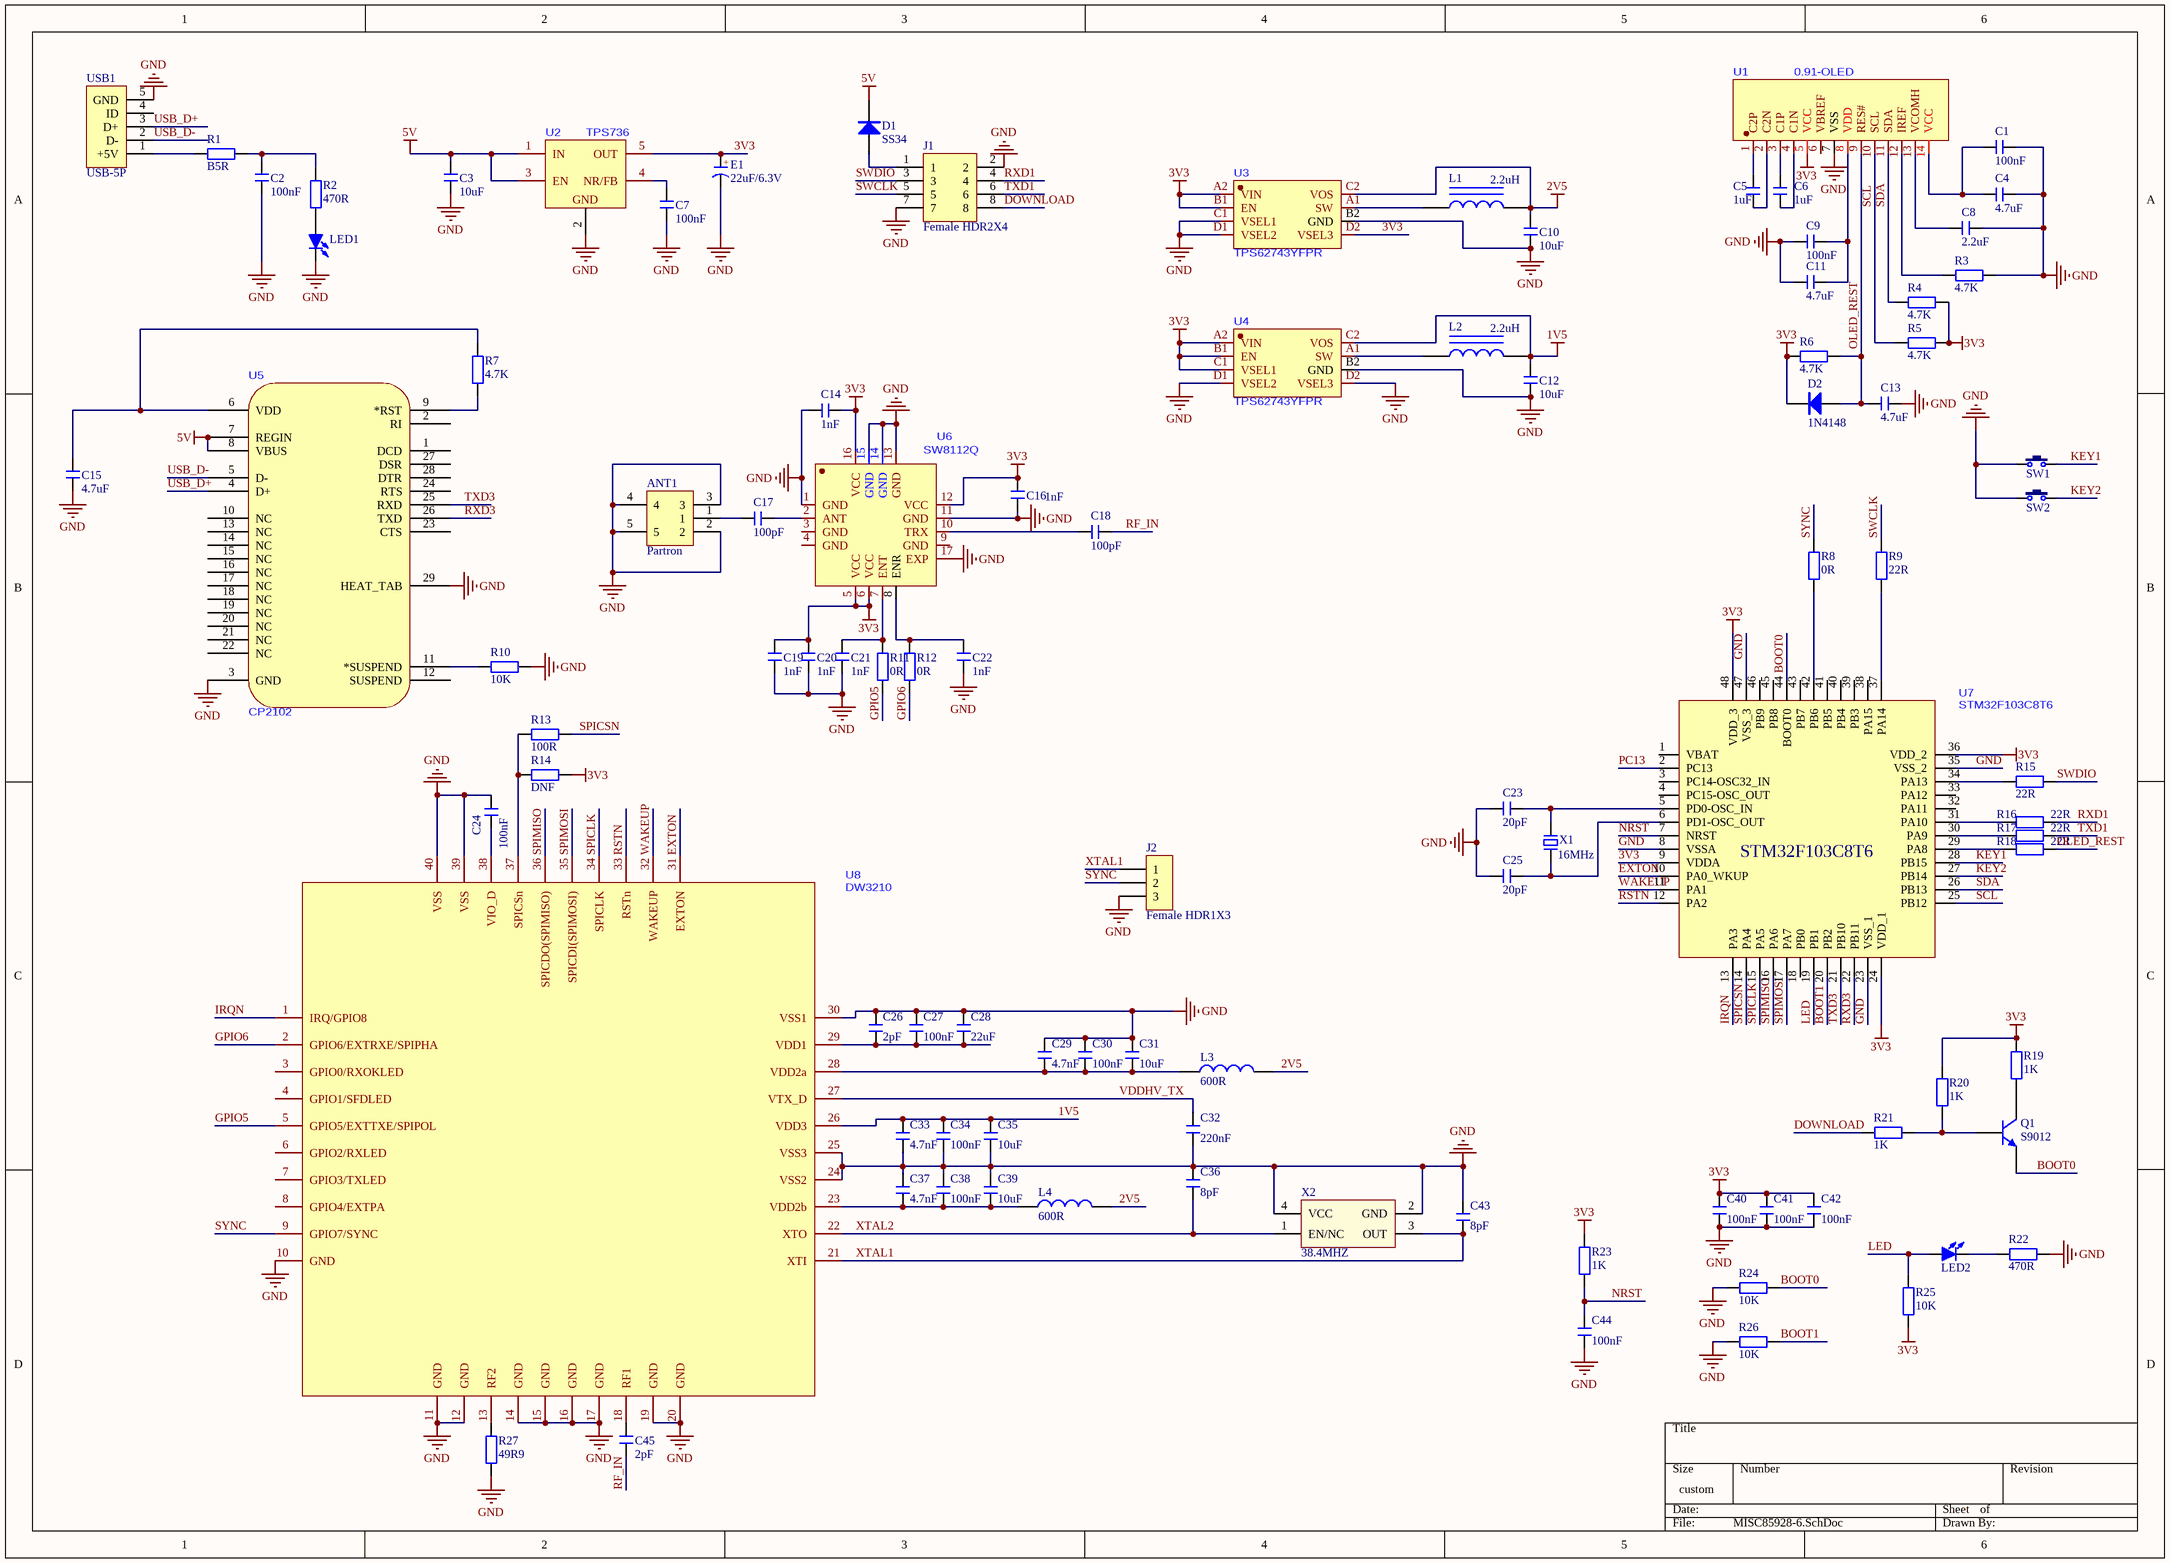
[diagram p0: MISC85928-6.SchDoc]
# Altium project MISC85928-2.PrjPcb
1 sheet, 98 parts. Net scope: global (net labels, ports and power ports of the same name join across sheets).
Board file: MISC85928.PcbDoc

## Sheet MISC85928-6.SchDoc
size 406 x 292 mm

### Parts
ANT1  Partron  [天线座5p]
C1  100nF  [C 0603_L]
C2  100nF  [C 0603_L]
C3  10uF  [C 0603_L]
C4  4.7uF  [C 0603_L]
C5  1uF  [C 0603_L]
C6  1uF  [C 0603_L]
C7  100nF  [C 0603_L]
C8  2.2uF  [C 0603_L]
C9  100nF  [C 0603_L]
C10  10uF  [C 0603_L]
C11  4.7uF  [C 0603_L]
C12  10uF  [C 0603_L]
C13  4.7uF  [C 0603_L]
C14  1nF  [C 0603_L]
C15  4.7uF  [C 0603_L]
C16  1nF  [C 0603_L]
C17  100pF  [C 0603_L]
C18  100pF  [C 0603_L]
C19  1nF  [C 0603_L]
C20  1nF  [C 0603_L]
C21  1nF  [C 0603_L]
C22  1nF  [C 0603_L]
C23  20pF  [C 0603_L]
C24  100nF  [C 0603_L]
C25  20pF  [C 0603_L]
C26  2pF  [C 0603_L]
C27  100nF  [C 0603_L]
C28  22uF  [C 0603_L]
C29  4.7nF  [C 0603_L]
C30  100nF  [C 0603_L]
C31  10uF  [C 0603_L]
C32  220nF  [C 0603_L]
C33  4.7nF  [C 0603_L]
C34  100nF  [C 0603_L]
C35  10uF  [C 0603_L]
C36  8pF  [C 0603_L]
C37  4.7nF  [C 0603_L]
C38  100nF  [C 0603_L]
C39  10uF  [C 0603_L]
C40  100nF  [C 0603_L]
C41  100nF  [C 0603_L]
C42  100nF  [C 0603_L]
C43  8pF  [C 0603_L]
C44  100nF  [C 0603_L]
C45  2pF  [C 0603_L]
D1  SS34  [MINI_MELF (LL34)]
D2  1N4148  [MINI_MELF (LL34)]
E1  22uF/6.3V  [C 0603_L]
J1  Female HDR2X4  [Fe-HDR2X4/2.54-S]
J2  Female HDR1X3  [Fe-HDR1X3/2.54-S]
L1  value 2.2uH  [L 0603]  (hidden comment: Inductor Iron)
L2  value 2.2uH  [L 0603]  (hidden comment: Inductor Iron)
L3  600R  [L 0603]
L4  600R  [L 0603]
LED1  Red  [LED 0805G]  (value not drawn)
LED2  Red  [LED 0805G]  (value not drawn)
Q1  S9012  [SOT-23B_N]
R1  B5R  [R 0603_L]
R2  470R  [R 0603_L]
R3  4.7K  [R 0603_L]
R4  4.7K  [R 0603_L]
R5  4.7K  [R 0603_L]
R6  4.7K  [R 0603_L]
R7  4.7K  [R 0603_L]
R8  0R  [R 0603_L]
R9  22R  [R 0603_L]
R10  10K  [R 0603_L]
R11  0R  [R 0603_L]
R12  0R  [R 0603_L]
R13  100R  [R 0603_L]
R14  DNF  [R 0603_L]
R15  22R  [R 0603_L]
R16  22R  [R 0603_L]
R17  22R  [R 0603_L]
R18  22R  [R 0603_L]
R19  1K  [R 0603_L]
R20  1K  [R 0603_L]
R21  1K  [R 0603_L]
R22  470R  [R 0603_L]
R23  1K  [R 0603_L]
R24  10K  [R 0603_L]
R25  10K  [R 0603_L]
R26  10K  [R 0603_L]
R27  49R9  [R 0603_L]
SW1  3x6x5  [TSW SMD-3*6*2.5]  (value not drawn)
SW2  3x6x5  [TSW SMD-3*6*2.5]  (value not drawn)
U1  0.91-OLED  [OLED0.91]
U2  TPS736  [SOT-23-5_L3.0-W1.7-P0.95-LS2.8-BR]
U3  TPS62743YFPR  [DSBGA-8_L1.6-W0.9-R2-C4-P0.40-BL]
U4  TPS62743YFPR  [DSBGA-8_L1.6-W0.9-R2-C4-P0.40-BL]
U5  CP2102  [CP2102]
U6  SW8112Q  [QFN-16_L3.0-W3.0-P0.50-BL-EP1.7]
U7  STM32F103C8T6  [LQFP48 7X7]
U8  DW3210  [DW3210]
USB1  USB-5P  [USB-MICRO_A]
X1  16MHz  [OSC 3215-2P]
X2  38.4MHZ  [OSC 1612-4P]

### Nets
1V5: C12.2 C33.1 C34.1 C35.1 L2.2 U4.C2(VOS) U8.26(VDD3)
2V5: C10.2 L1.2 L3.2 L4.2 U3.C2(VOS)
3V3: C14.1 C16.1 C19.1 C20.1 C40.1 C41.1 C42.1 D2.2(K) E1.1(A) R4.1 R5.1 R6.2 R14.1 R19.1 R20.1 R23.2 R25.2 U1.5(VCC) U2.5(OUT) U3.A2(VIN) U3.B1(EN) U3.D2(VSEL3) U4.A2(VIN) U4.B1(EN) U4.C1(VSEL1) U6.5(VCC) U6.6(VCC) U6.12(VCC) U6.16(VCC) U7.9(VDDA) U7.24(VDD_1) U7.36(VDD_2) U7.48(VDD_3)
5V: C3.2 D1.2(K) U2.1(IN) U2.3(EN) U5.7(REGIN) U5.8(VBUS)
GND: ANT1.2 ANT1.3 ANT1.4 ANT1.5 C1.1 C2.1 C3.1 C4.1 C7.1 C8.1 C9.2 C10.1 C11.2 C12.1 C13.1 C14.2 C15.1 C16.2 C19.2 C20.2 C21.2 C22.2 C23.1 C24.1 C25.1 C26.1 C27.1 C28.1 C29.1 C30.1 C31.1 C32.2 C33.2 C34.2 C35.2 C36.1 C37.1 C38.1 C39.1 C40.2 C41.2 C42.2 C43.1 C44.2 E1.2(K) J1.2 J1.7 J2.3 LED1.2(K) R3.1 R10.1 R22.2 R24.2 R26.2 R27.1 SW1.1 SW2.1 U1.7(VSS) U2.2(GND) U3.B2(GND) U3.C1(VSEL1) U3.D1(VSEL2) U4.B2(GND) U4.D1(VSEL2) U4.D2(VSEL3) U5.3(GND) U5.29(HEAT_TAB) U6.1(GND) U6.11(GND) U6.13(GND) U6.14(GND) U6.15(GND) U6.17(EXP) U7.8(VSSA) U7.23(VSS_1) U7.35(VSS_2) U7.47(VSS_3) U8.10(GND) U8.11(GND) U8.12(GND) U8.14(GND) U8.15(GND) U8.16(GND) U8.17(GND) U8.19(GND) U8.20(GND) U8.24(VSS2) U8.25(VSS3) U8.30(VSS1) U8.39(VSS) U8.40(VSS) USB1.5(GND) X2.2(GND) X2.4(VCC)
BOOT0: Q1.3(E) R24.1 U7.44(BOOT0)
BOOT1: R26.1 U7.20(PB2)
DOWNLOAD: J1.8 R21.1
EXTON: U7.10(PA0_WKUP) U8.31(EXTON)
GPIO5: R11.1 U8.5(GPIO5/EXTTXE/SPIPOL)
GPIO6: R12.1 U8.2(GPIO6/EXTRXE/SPIPHA)
IRQN: U7.13(PA3) U8.1(IRQ/GPIO8)
KEY1: SW1.2 U7.28(PB15)
KEY2: SW2.2 U7.27(PB14)
LED: LED2.1(A) R25.1 U7.19(PB1)
NRST: C44.1 R23.1 U7.7(NRST)
OLED_REST: C13.2 D2.1(A) R6.1 R18.1 U1.9(RES#)
PC13: U7.2(PC13)
RF_IN: C18.1 C45.2
RSTN: U7.12(PA2) U8.33(RSTn)
RXD1: J1.4 R16.1
RXD3: U5.26(TXD) U7.22(PB11)
SCL: R5.2 U1.10(SCL) U7.25(PB12)
SDA: R4.2 U1.11(SDA) U7.26(PB13)
SPICLK: U7.15(PA5) U8.34(SPICLK)
SPICSN: R13.1 U7.14(PA4)
SPIMISO: U7.16(PA6) U8.36(SPICDO(SPIMISO))
SPIMOSI: U7.17(PA7) U8.35(SPICDI(SPIMOSI))
SWCLK: J1.5 R9.2
SWDIO: J1.3 R15.1
SYNC: J2.2 R8.2 U8.9(GPIO7/SYNC)
TXD1: J1.6 R17.1
TXD3: U5.25(RXD) U7.21(PB10)
USB_D+: U5.4(D+) USB1.3(D+)
USB_D-: U5.5(D-) USB1.2(D-)
VDDHV_TX: C32.1 U8.27(VTX_D)
WAKEUP: U7.11(PA1) U8.32(WAKEUP)
XTAL1: C43.2 J2.1 U8.21(XTI) X2.3(OUT)
XTAL2: C36.2 U8.22(XTO) X2.1(EN/NC)
NetANT1_1: ANT1.1 C17.2
NetC1_2: C1.2 C4.2 U1.14(VCC)
NetC2_2: C2.2 R1.2 R2.2
NetC5_1: C5.1 U1.2(C2N)
NetC5_2: C5.2 U1.1(C2P)
NetC6_1: C6.1 U1.4(C1N)
NetC6_2: C6.2 U1.3(C1P)
NetC7_2: C7.2 U2.4(NR/FB)
NetC8_2: C8.2 U1.13(VCOMH)
NetC9_1: C9.1 C11.1 U1.8(VDD)
NetC15_2: C15.2 R7.2 U5.6(VDD)
NetC17_1: C17.1 U6.2(ANT)
NetC18_2: C18.2 U6.10(TRX)
NetC21_1: C21.1 R11.2 U6.7(ENT)
NetC22_1: C22.1 R12.2 U6.8(ENR)
NetC23_2: C23.2 U7.5(PD0-OSC_IN) X1.2
NetC24_2: C24.2 U8.38(VIO_D)
NetC25_2: C25.2 U7.6(PD1-OSC_OUT) X1.1
NetC26_2: C26.2 C27.2 C28.2 U8.29(VDD1)
NetC29_2: C29.2 C30.2 C31.2 L3.1 U8.28(VDD2a)
NetC37_2: C37.2 C38.2 C39.2 L4.1 U8.23(VDD2b)
NetC45_1: C45.1 U8.18(RF1)
NetD1_1: D1.1(A) J1.1
NetL1_1: L1.1 U3.A1(SW)
NetL2_1: L2.1 U4.A1(SW)
NetLED1_1: LED1.1(A) R2.1
NetLED2_2: LED2.2(K) R22.1
NetQ1_1: Q1.1(C) R19.2
NetQ1_2: Q1.2(B) R20.2 R21.2
NetR1_1: R1.1 USB1.1(+5V)
NetR3_2: R3.2 U1.12(IREF)
NetR7_1: R7.1 U5.9(*RST)
NetR8_1: R8.1 U7.42(PB6)
NetR9_1: R9.1 U7.37(PA14)
NetR10_2: R10.2 U5.11(*SUSPEND)
NetR13_2: R13.2 R14.2 U8.37(SPICSn)
NetR15_2: R15.2 U7.34(PA13)
NetR16_2: R16.2 U7.31(PA10)
NetR17_2: R17.2 U7.30(PA9)
NetR18_2: R18.2 U7.29(PA8)
NetR27_2: R27.2 U8.13(RF2)

Not connected (* = marked no-connect by the designer): U1 6(VBREF); U5 1(DCD) 2(RI) 10(NC) 12(SUSPEND) 13(NC) 14(NC) 15(NC) 16(NC) 17(NC) 18(NC) 19(NC) 20(NC) 21(NC) 22(NC) 23(CTS) 24(RTS) 27(DSR) 28(DTR); U6 3(GND) 4(GND) 9(GND); U7 1(VBAT) 3(PC14-OSC32_IN) 4(PC15-OSC_OUT) 18(PB0) 32(PA11) 33(PA12) 38(PA15) 39(PB3) 40(PB4) 41(PB5) 43(PB7) 45(PB8) 46(PB9); U8 3(GPIO0/RXOKLED) 4(GPIO1/SFDLED) 6(GPIO2/RXLED) 7(GPIO3/TXLED) 8(GPIO4/EXTPA); USB1 4(ID)

### Library data of the parts
C1-C45 = C: Chip capacitor; BOM名称: Non-polar chip capacitor
D1 D2 = 1N4148: Switching diode; BOM名称: High-speed switching diode
E1 = CT: Chip tantalum capacitor; BOM名称: Chip tantalum capacitor
L1 L2 = Inductor Iron: Magnetic-Core Inductor; Published: 24-Mar-1999; LatestRevisionDate: 17-Jul-2002; LatestRevisionNote: Re-released for DXP Platform.; PackageReference: AXIAL-0.9; PackageDescription: Axial Device, Thru-Hole; 2 Leads; 0.9 in Pin Spacing; Publisher: Altium Limited
L3 L4 = L: Low-power chip inductor; BOM名称: Low-power chip inductor
LED1 LED2 = LED-SMD: Chip LED; BOM名称: Chip LED
Q1 = QNPN: NPN Bipolar Transistor; Published: 8-Jun-2000; LatestRevisionDate: 29-May-2009; LatestRevisionNote: IPC-7351 Footprint Added.; PackageVersion: Aug-1999; PackageReference: SOT-23B; PackageDescription: 3-Pin SOT-23 Package 0.95 mm Pitch, 2.4 mm Lead Span; Publisher: Altium Limited
R1-R27 = R: Chip resistor; BOM名称: Chip resistor
SW1 SW2 = TSW 3x6: 3x6 tact switch; BOM名称: 3x6 tact switch
U2 = TPS73633DBVR
U5 = CP2102_1
USB1 = USB-5P: Micro USB female socket; BOM名称: Micro USB female socket
X1 = XTAL-2P: 2-pin passive crystal; BOM名称: 2-pin passive crystal
X2 = XTAL-ACT-4P: 4-pin active crystal oscillator; BOM名称: 4-pin active crystal oscillator